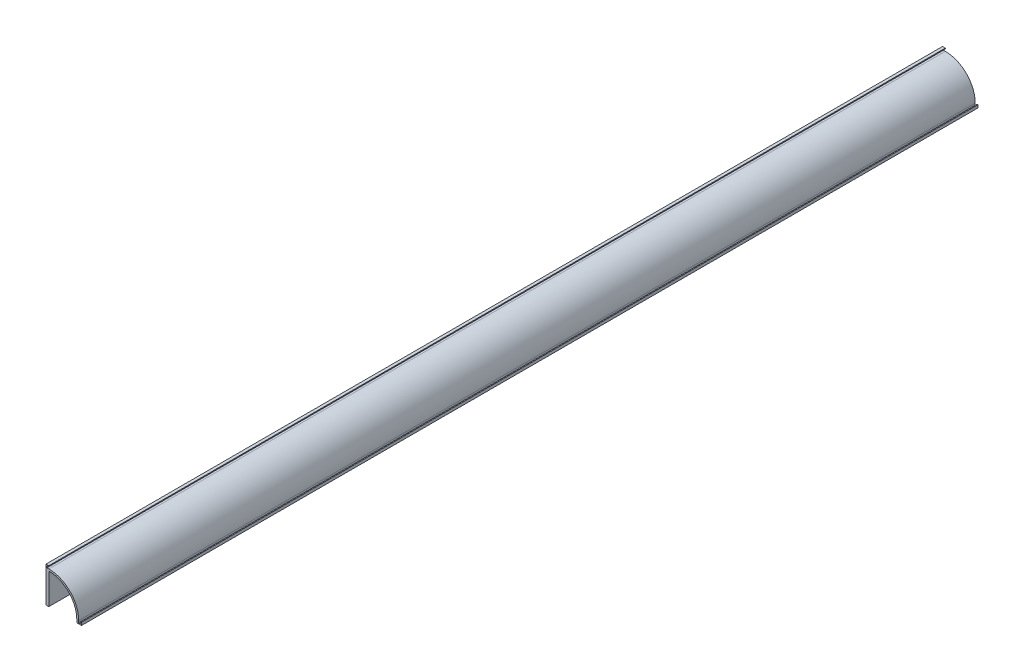
SolidWorks part; units mm, degrees
ref_plane "Frontal" through (0, 0, 0) normal (0, 0, 1) x (1, 0, 0)
ref_plane "Superior" through (0, 0, 0) normal (0, 1, 0) x (1, 0, 0)
ref_plane "Direito" through (0, 0, 0) normal (1, 0, 0) x (0, 0, -1)
sketch "Sketch1" plane through (0, 0, 0) normal (0, 0, 1) x (1, 0, 0)
  line L0 (0, 0) -> (0, 19)
  line L1 (0, 19) -> (1.5, 19)
  line L2 (1.5, 19) -> (1.5, 18.5)
  line L3 (1.5, 18.5) -> (0.5, 18.5)
  line L4 (0.5, 18.5) -> (0.5, 17.5)
  line L5 (0.5, 17.5) -> (1.5, 17.5)
  line L6 (17.5, 1.5) -> (17.5, 0.5)
  line L7 (17.5, 0.5) -> (18.5, 0.5)
  line L8 (18.5, 0.5) -> (18.5, 1.5)
  line L9 (18.5, 1.5) -> (19, 1.5)
  line L10 (0, 0) -> (1.5, 0)
  line L11 (1.5, 0) -> (1.5, 16.5)
  line L12 (16.5, 1.5) -> (16.5, 0)
  line L13 (16.5, 0) -> (19, 0)
  line L14 (19, 0) -> (19, 1.5)
  arc A0 (1.5, 17.5) -> (17.5, 1.5) centre (1.5, 1.5) cw
  arc A1 (1.5, 16.5) -> (16.5, 1.5) centre (1.5, 1.5) cw
  dimension "D6" = 1
  dimension "D10" = 15
  dimension "D1" = 1.5
  dimension "D2" = 1.5
  dimension "D3" = 0.5
  dimension "D4" = 1
  dimension "D5" = 1
  dimension "D7" = 1.5
  dimension "D8" = 2.5
  dimension "D9" = 1
  dimension "D11" = 1
  dimension "D12" = 1
extrude "Boss-Extrude1" add sketch "Sketch1" along normal blind 480
